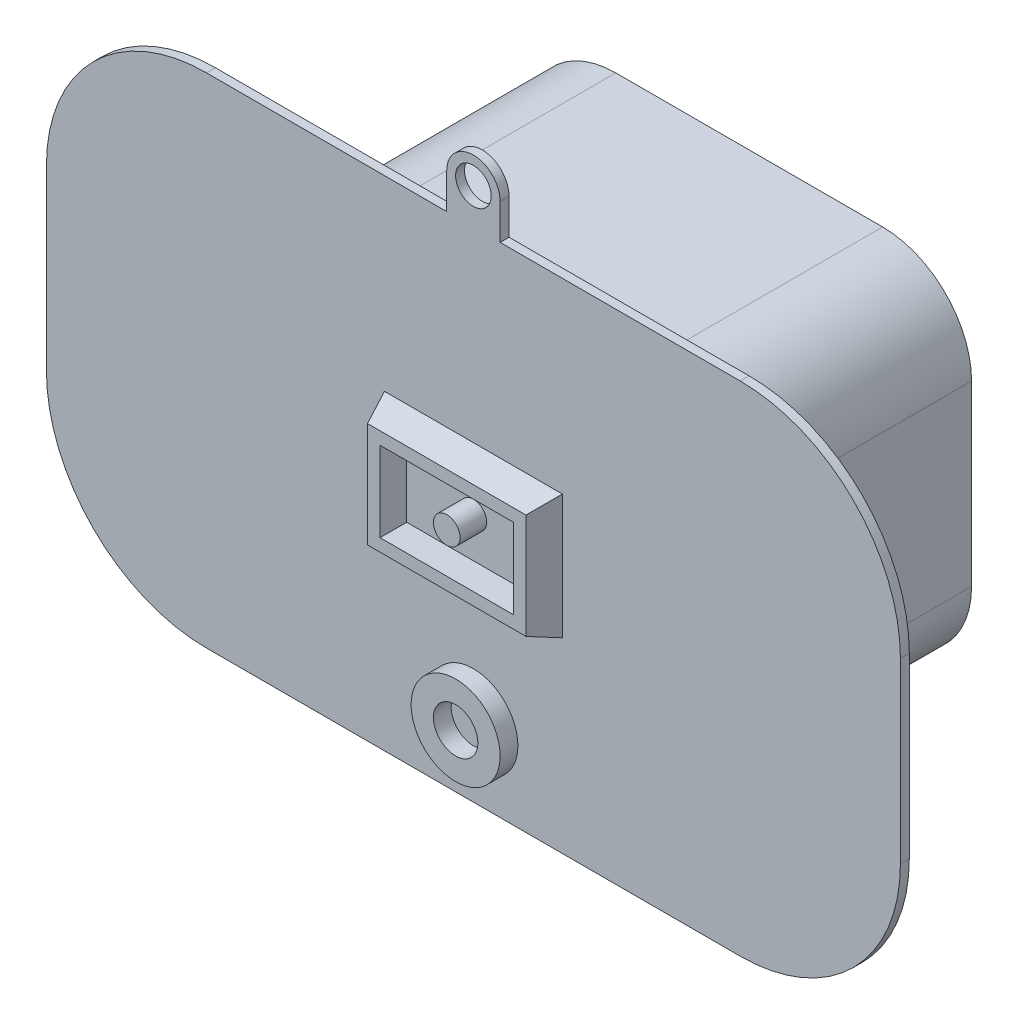
SolidWorks part; units mm, degrees
ref_plane "Front Plane" through (0, 0, 0) normal (0, 0, 1) x (1, 0, 0)
ref_plane "Top Plane" through (0, 0, 0) normal (0, 1, 0) x (1, 0, 0)
ref_plane "Right Plane" through (0, 0, 0) normal (1, 0, 0) x (0, 0, -1)
sketch "Sketch1" plane through (0, 0, 0) normal (0, 0, 1) x (1, 0, 0)
  line L0 (-3, 28) -> (-3, 32)
  line L1 (-30, 28) -> (-3, 28)
  line L2 (-48, 10) -> (-48, -10)
  line L3 (-30, -28) -> (30, -28)
  line L4 (48, 10) -> (48, -10)
  line L5 (-48, 28) -> (48, -28) construction
  line L6 (-48, -28) -> (48, 28) construction
  line L7 (3, 32) -> (3, 28)
  line L8 (3, 28) -> (30, 28)
  arc A0 (-48, -10) -> (-30, -28) centre (-30, -10) ccw
  arc A1 (30, -28) -> (48, -10) centre (30, -10) ccw
  arc A2 (30, 28) -> (48, 10) centre (30, 10) cw
  arc A3 (-30, 28) -> (-48, 10) centre (-30, 10) ccw
  arc A4 (-3, 32) -> (3, 32) centre (0, 32) cw
  circle A5 centre (0, 32) radius 2
  point P0 (0, 0)
  dimension "D3" = 18
  dimension "D4" = 4
  dimension "D6" = 3
  dimension "D1" = 96
  dimension "D2" = 56
  dimension "D5" = 4
extrude "Boss-Extrude1" add sketch "Sketch1" along normal blind 1
sketch "Sketch2" plane through (0, 0, 1) normal (0, 0, 1) x (1, 0, 0)
  line L1 (-10, 7) -> (10, 7)
  line L2 (-10, 7) -> (-10, -7)
  line L3 (-10, -7) -> (10, -7)
  line L4 (10, 7) -> (10, -7)
  line L5 (-10, 7) -> (10, -7) construction
  line L6 (-10, -7) -> (10, 7) construction
  point P0 (0, 0)
  dimension "D1" = 14
  dimension "D2" = 20
extrude "Boss-Extrude2" add sketch "Sketch2" along normal blind 3 draft 20
sketch "Sketch3" plane through (0, 0, 4) normal (0, 0, 1) x (1, 0, 0)
  line L1 (-7.5, 4.5) -> (7.5, 4.5)
  line L2 (-7.5, 4.5) -> (-7.5, -4.5)
  line L3 (-7.5, -4.5) -> (7.5, -4.5)
  line L4 (7.5, 4.5) -> (7.5, -4.5)
  line L5 (-7.5, 4.5) -> (7.5, -4.5) construction
  line L6 (-7.5, -4.5) -> (7.5, 4.5) construction
  circle A0 centre (0, 0) radius 1.5
  dimension "D3" = 3
  dimension "D1" = 15
  dimension "D2" = 9
extrude "Cut-Extrude1" cut sketch "Sketch3" against normal blind 3
sketch "Sketch4" plane through (0, 0, 0) normal (0, 0, -1) x (-1, 0, 0)
  line L1 (-25, 20) -> (25, 20)
  line L2 (-25, 20) -> (-25, -20)
  line L3 (-25, -20) -> (25, -20)
  line L4 (25, 20) -> (25, -20)
  line L5 (-25, 20) -> (25, -20) construction
  line L6 (-25, -20) -> (25, 20) construction
  line L7 (-23, 18) -> (23, 18)
  line L8 (-23, 18) -> (-23, -18)
  line L9 (-23, -18) -> (23, -18)
  line L10 (23, 18) -> (23, -18)
  line L11 (-23, 18) -> (23, -18) construction
  line L12 (-23, -18) -> (23, 18) construction
  point P0 (0, 0)
  point P6 (0, 0)
  dimension "D1" = 50
  dimension "D2" = 40
  dimension "D3" = 2
  dimension "D4" = 2
extrude "Boss-Extrude3" add sketch "Sketch4" along normal blind 30
sketch "Sketch5" plane through (0, 0, 1) normal (0, 0, 1) x (1, 0, 0)
  circle A0 centre (0, -20) radius 5
  circle A1 centre (0, -20) radius 2.5
  dimension "D1" = 10
  dimension "D3" = 5
  dimension "D2" = 20
extrude "Boss-Extrude4" add sketch "Sketch5" along normal blind 2
fillet "Fillet1" radius 8 4 edges at (23, 18, -15) (-23, 18, -15) (-23, -18, -15) (23, -18, -15)
fillet "Fillet2" radius 10 4 edges at (25, 20, -15) (25, -20, -15) (-25, 20, -15) (-25, -20, -15)
